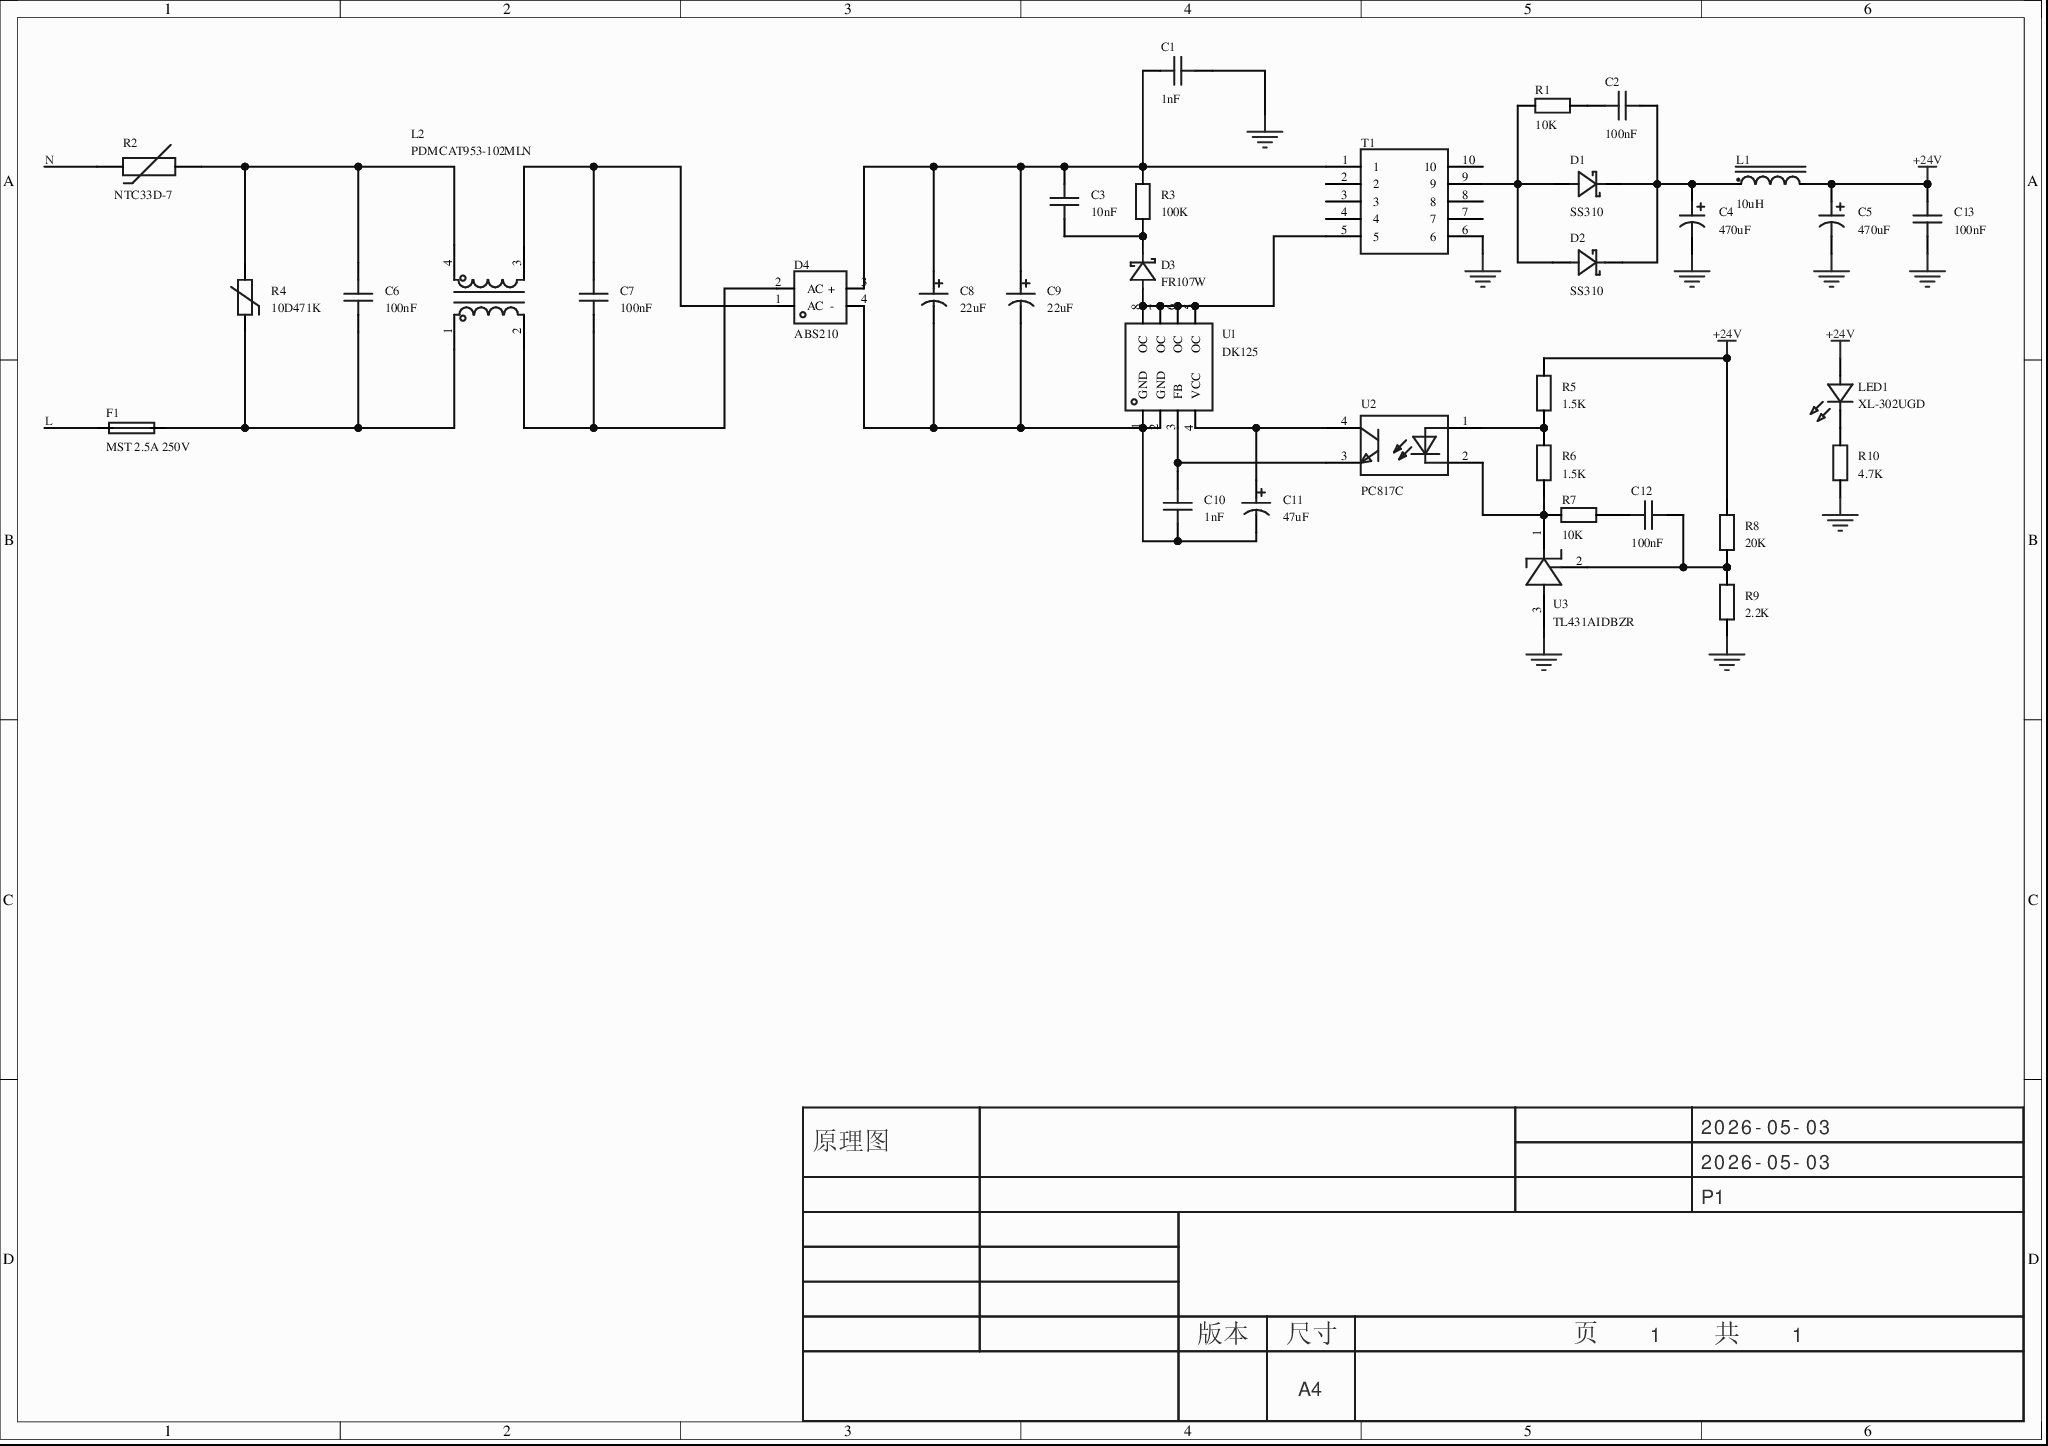
[diagram p0: MISC51479-3.schdoc]
# Altium project MISC51479-2.PrjPcb
1 sheet, 35 parts. Net scope: global (net labels, ports and power ports of the same name join across sheets).
Board file: MISC51479.pcbdoc

## Sheet MISC51479-3.schdoc
size 297 x 209 mm; Version: V1.0; @Project Name: MISC51479; @Page Count: 1; @Update Date: 2026-05-03; @Create Date: 2026-05-03; @Schematic Name: MISC51479; @Page No: 1; @Create Time: 01:06:52; @Update Time: 01:06:58; @Board Name: MISC51479

### Parts
C1  1nF  [CAP-TH_L7.5-W4.5-P10.00-D0.6]
C2  100nF  [C0603]
C3  10nF  [C1206]
C4  470uF  [CAP-TH_BD8.0-P3.50-D0.6-FD]
C5  470uF  [CAP-TH_BD8.0-P3.50-D0.6-FD]
C6  100nF  [CAP-TH_L13.0-W6.0-P10.00-D0.6]
C7  100nF  [CAP-TH_L13.0-W6.0-P10.00-D0.6]
C8  22uF  [CAP-TH_BD10.0-P5.00-D1.0-FD]
C9  22uF  [CAP-TH_BD10.0-P5.00-D1.0-FD]
C10  1nF  [C0603]
C11  47uF  [CAP-TH_BD5.0-P2.00-D0.8-FD]
C12  100nF  [C0603]
C13  100nF  [C0603]
D1  SS310  [SMA_L4.3-W2.6-LS5.0-FD]
D2  SS310  [SMA_L4.3-W2.6-LS5.0-FD]
D3  FR107W  [SOD-123FL_L2.7-W1.8-LS3.8-RD]
D4  ABS210  [ABF_L5.1-W4.4-P4.00-LS6.2-BL]
F1  MST 2.5A 250V  [FUSE-TH_L8.4-W4.3-P5.08-D1.0]
L1  10uH  [IND-TH_BD8.0-P5.00-D0.7]
L2  PDMCAT953-102MLN  [IND-TH_4P-L12.0-W6.0_PDMCAT953-501MLN]
LED1  XL-302UGD  [LED-TH_BD3.8-P2.54-FD_GREEN]
R1  10K  [R0603]
R2  NTC33D-7  [RES-TH_L6.5-W5.0-P5.00-D0.6-S4.40]
R3  100K  [R1206]
R4  10D471K  [RES-TH_L11.0-W6.0-P7.50-D0.8-S3.00]
R5  1.5K  [R0603]
R6  1.5K  [R0603]
R7  10K  [R0603]
R8  20K  [R0603]
R9  2.2K  [R0603]
R10  4.7K  [R0603]
T1  (no value)  [EE25 5+5]
U1  DK125  [DIP-8_L9.2-W6.4-P2.54-LS7.6-BL]
U2  PC817C  [DIP-4_L4.6-W6.5-P2.54-LS7.6-BL]
U3  TL431AIDBZR  [SOT-23-3_L2.9-W1.6-P1.90-LS2.8-BR]

### Nets
+24V: C5.1 C13.2 L1.2 LED1.1(A) R5.2 R8.2
GND: C1.2 C4.2 C5.2 C13.1 R9.1 R10.1 T1.6 U3.3(ANODE)
L: F1.1
N: R2.1
NetC1_1: C1.1 C3.2 C8.1 C9.1 D4.3(+) R3.2 T1.1
NetC2_1: C2.1 R1.2
NetC2_2: C2.2 C4.1 D1.2(K) D2.2(K) L1.1
NetC3_1: C3.1 D3.1(K) R3.1
NetC6_1: C6.1 L2.4 R2.2 R4.2
NetC6_2: C6.2 F1.2 L2.1 R4.1
NetC7_1: C7.1 D4.1(AC) L2.3
NetC7_2: C7.2 D4.2(AC) L2.2
NetC8_2: C8.2 C9.2 C10.1 C11.2 D4.4(-) U1.1(GND) U1.2(GND)
NetC10_2: C10.2 U1.3(FB) U2.3(EM)
NetC11_1: C11.1 U1.4(VCC) U2.4(COL)
NetC12_1: C12.1 R8.1 R9.2 U3.2(REF)
NetC12_2: C12.2 R7.2
NetD1_1: D1.1(A) D2.1(A) R1.1 T1.9
NetD3_2: D3.2(A) T1.5 U1.5(OC) U1.6(OC) U1.7(OC) U1.8(OC)
NetLED1_2: LED1.2(K) R10.2
NetR5_1: R5.1 R6.2 U2.1(AN)
NetR6_1: R6.1 R7.1 U2.2(CAT) U3.1(CATHODE)

Not connected (* = marked no-connect by the designer): T1 2* 3* 4* 7* 8* 10

### Notes on the sheet
- 2026-05-03
- 原理图
- P1
- 版本
- 尺寸
- A4
- 页    1    共    1

### Library data of the parts
C1 = KY1102M400VAC70Y10093: 容值:1nF;精度:±20%;工作电压(AC):400V;防护等级:Y1;; Manufacturer: KNSCHA(科尼盛); AddInBom: yes; ModelId: 9383b9b23f884ae7b98244ec8344dac5; ModelTransform: 431.76158,177.165,0,0,0,0,0,0,-137.795; Tolerance: ±20%; Voltage(AC): 400V; Ratings: Y1; safety certification: UL；ENEC；VDE；CQC; Symbol: KY1102M400VAC70Y10093; Device: KY1102M400VAC70Y10093; LCSC Part Name: 1nF ±20% 400V 等级:Y1; SupplierPart: C2943996; ManufacturerPart: KY1102M400VAC70Y10093; Supplier Footprint: 插件,P=10mm; JLCPCB Part Class: 扩展库; Datasheet: https://atta.szlcsc.com/upload/public/pdf/source/20240902/B2C4860AD6BBA55A7E27F7C368C73C02.pdf; Supplier: LCSC; ConvertToPcb: yes; FootprintName: CAP-TH_L7.5-W4.5-P10.00-D0.6; ModelName: CAP-TH_L7.5-W4.5-P10.00-D0.6; Value: 1nF
C2 C3 C10 C12 C13 = CAP_0603: ConvertToPcb: yes; SymbolName: Capacitance; ModelId: ac125912035d415993ca9572d50418b1; ModelName: C0603_L1.6-W0.8-H0.8; ModelTransform: 62.992,31.496,0,0,0,0,0,0,0; Device: CAP_0603; AddInBom: yes; Supplier Footprint: 0603
  C2 C12 C13: FootprintName: C0603; Value: 100nF
  C3: Value: 10nF; FootprintName: C1206
  C10: Value: 1nF; FootprintName: C0603
C4 C5 = JBLH2471M035D140RLM 470UF 35V: 容值:470uF;精度:±20%;额定电压:35V;纹波电流:2.9A@100kHz;等效串联电阻(ESR):35mΩ@100kHz;; Manufacturer: DMBJ(振宝佳); AddInBom: yes; ModelId: a2c936ec27754f809f3966430e36f767; ModelName: CAP-TH_D8.0-H8.0-P3.50; ModelTransform: 314.96,314.862,0,180,0,0,0,0,-137.795; Tolerance: ±20%; Voltage Rating: 35V; Lifetime: 2000hrs@105℃; Symbol: JBLH2471M035D140RLM 470UF 35V; Device: JBLH2471M035D140RLM 470UF 35V; LCSC Part Name: 470uF ±20% 35V; SupplierPart: C19270680; ManufacturerPart: JBLH2471M035D140RLM 470UF 35V; Supplier Footprint: 插件,D8xL14mm; JLCPCB Part Class: 扩展库; Datasheet: https://item.szlcsc.com/datasheet/JBLH2471M035D140RLM%2520470UF%252035V/20537870.html; Supplier: LCSC; ConvertToPcb: yes; FootprintName: CAP-TH_BD8.0-P3.50-D0.6-FD; Value: 470uF; Ripple Current: 2.9A@100kHz; Equivalent Series Resistance(ESR): 35mΩ@100kHz; Diameter: 8mm; Height - Seated (Max): 14mm
C6 C7 = MPX104K31C3KN15600: 容值:100nF;精度:±10%;工作电压(AC):275V；310V；305V;防护等级:X2;; Manufacturer: KNSCHA(科尼盛); AddInBom: yes; ModelId: ab2ba9e918834f5e935e28a3e5a6a2b8; ModelName: CAP-TH_L13.0-W6.0-H12.0-P10.0; ModelTransform: 511.81,236.22,0,0,0,0,0,0,-137.795; Tolerance: ±10%; Ratings: X2; safety certification: UL；CUL；KC；ENEC；VDE；CQC; Symbol: MPX104K31C3KN15600; Device: MPX104K31C3KN15600; LCSC Part Name: 100nF ±10% 275V 305V 310V 等级:X2; SupplierPart: C489079; ManufacturerPart: MPX104K31C3KN15600; Supplier Footprint: 插件,P=10mm; JLCPCB Part Class: 扩展库; Datasheet: https://atta.szlcsc.com/upload/public/pdf/source/20200225/C489079_75CB6A5338414DC85C4C6073302579B5.pdf; Supplier: LCSC; ConvertToPcb: yes; FootprintName: CAP-TH_L13.0-W6.0-P10.00-D0.6; Value: 100nF; Voltage(AC): 275V；310V；305V; Operating Temperature: -40℃~+110℃
C8 C9 = ERK2GM220G16OT: 容值:22uF;精度:±20%;额定电压:400V;纹波电流:-;等效串联电阻(ESR):-;; Manufacturer: AISHI(艾华集团); AddInBom: yes; ModelId: 6ce78ce5315348e095d700085da75e48; ModelName: CAP-TH_D10.0-H16.0-P5.00; ModelTransform: 394.094,393.72252,0,0,0,0,0,0,-137.795; Tolerance: ±20%; Voltage Rating: 400V; Pin Spacing: 5mm; Lifetime: 2000hrs@105℃; Symbol: ERK2GM220G16OT; Device: ERK2GM220G16OT; LCSC Part Name: 22uF ±20% 400V CLEAR 专门用于充电器; SupplierPart: C106587; ManufacturerPart: ERK2GM220G16OT; Supplier Footprint: 插件,D10xL16mm; JLCPCB Part Class: 扩展库; Datasheet: https://item.szlcsc.com/datasheet/ERK2GM220G16OT/107803.html; Supplier: LCSC; ConvertToPcb: yes; FootprintName: CAP-TH_BD10.0-P5.00-D1.0-FD; Value: 22uF; Ripple Current: -; Equivalent Series Resistance(ESR): -; Diameter: 10mm; Height - Seated (Max): 16mm
C11 = KS476M025D07RR0VH2FP0: 容值:47uF;精度:±20%;额定电压:25V;; Manufacturer: Chengx(承兴); Symbol: 47uF 25V 5*7; AddInBom: yes; ModelId: edeeed87cbc746108d01291548c38636; ModelName: CAP-TH_D5.0×H7.0×P2.0; ModelTransform: 197.091,196.7911,0,0,0,0,0,0,-137.795; Tolerance: ±20%; Voltage Rating: 25V; Pin Spacing: 2mm; Lifetime: 1000hrs@105℃; Device: KS476M025D07RR0VH2FP0; LCSC Part Name: 47uF ±20% 25V; SupplierPart: C44586; ManufacturerPart: KS476M025D07RR0VH2FP0; Supplier Footprint: 插件,D5xL7mm; JLCPCB Part Class: 扩展库; Datasheet: https://item.szlcsc.com/datasheet/KS476M025D07RR0VH2FP0/45588.html; Supplier: LCSC; ConvertToPcb: yes; FootprintName: CAP-TH_BD5.0-P2.00-D0.8-FD; Value: 47uF; Diameter: 5mm; Height - Seated (Max): 7mm; Operating Temperature: -40℃~+105℃
D1 D2 = SS310_C7420364: 二极管配置:独立式;正向压降(Vf):850mV@3A;直流反向耐压(Vr):100V;整流电流:3A;; Manufacturer: R+O(宏嘉诚); AddInBom: yes; ModelId: 7e24bebe6cd74171ae8c9de6fc5b78aa; ModelTransform: 198.4248,103.5431,0,180,0,0,0,0,0; Diode Configuration: 独立式; Voltage - DC Reverse(Vr): 100V; Current - Rectified: 3A; Reverse Leakage Current (Ir): 50uA@100V; Operating Junction Temperature Range: -55℃~+150℃; Non-Repetitive Peak Forward Surge Current: 80A; Symbol: SS310_C7420364; Device: SS310_C7420364; LCSC Part Name: 电压:100V 电流:3A; SupplierPart: C7420364; ManufacturerPart: SS310; Supplier Footprint: SMA(DO-214AC); JLCPCB Part Class: 扩展库; Datasheet: https://item.szlcsc.com/datasheet/SS310/8397186.html; Supplier: LCSC; ConvertToPcb: yes; FootprintName: SMA_L4.3-W2.6-LS5.0-FD; ModelName: SMA_L4.3-W2.6-LS5.0-FD; Voltage - Forward(Vf@If): 850mV@3A
D3 = FR107W_C18199114: 二极管配置:独立式;正向压降(Vf):1.3V@1.0A;直流反向耐压(Vr):1kV;整流电流:1A;反向恢复时间(Trr):500ns;; Manufacturer: R+O(宏嘉诚); AddInBom: yes; ModelId: 86f9151e155e4fe2af0c4f2e0a80302e; ModelName: SOD-123FL_L2.8-W1.8-H1.1-LS3.6; ModelTransform: 141.732,70.866,0,180,0,0,0,0,0; Diode Configuration: 独立式; Voltage - DC Reverse(Vr): 1kV; Current - Rectified: 1A; Reverse Leakage Current (Ir): 2uA@1000V; Reverse Recovery Time (trr): 500ns; Operating Junction Temperature Range: -55℃~+150℃; Non-Repetitive Peak Forward Surge Current: 30A; Symbol: FR107W_C18199114; Device: FR107W_C18199114; LCSC Part Name: 耐压:1000V 电流:1A 反向恢复时间：500ns; SupplierPart: C18199114; ManufacturerPart: FR107W; Supplier Footprint: SOD-123FL; JLCPCB Part Class: 扩展库; Datasheet: https://item.szlcsc.com/datasheet/FR107W/19354346.html; Supplier: LCSC; ConvertToPcb: yes; FootprintName: SOD-123FL_L2.7-W1.8-LS3.8-RD; Voltage - Forward(Vf@If): 1.3V@1.0A
D4 = ABS210_C42406052: 正向压降(Vf):1V@1A;直流反向耐压(Vr):1kV;整流电流:2A;非重复峰值浪涌电流 (Ifsm):60A;; Manufacturer: R+O(宏嘉诚); AddInBom: yes; ModelId: d26de62a0ec4497f9836f9d57bcbc20d; ModelName: ABF_L5.1-W4.4-H1.1-LS6.2-P4.00; ModelTransform: 200.787,244.094,0,0,0,0,0,0,0; Voltage - Forward(Vf@If): 1V@1A; Voltage - DC Reverse(Vr): 1kV; Current - Rectified: 2A; Reverse Leakage Current (Ir): 5uA; Non-Repetitive Peak Forward Surge Current: 60A; Operating Junction Temperature Range: -55℃~+150℃; Symbol: ABS210_C42406052; Device: ABS210_C42406052; LCSC Part Name: 耐压:1000V 电流:2A; SupplierPart: C42406052; ManufacturerPart: ABS210; Supplier Footprint: ABS; JLCPCB Part Class: 扩展库; Datasheet: https://item.szlcsc.com/datasheet/ABS210/44376175.html; Supplier: LCSC; ConvertToPcb: yes; FootprintName: ABF_L5.1-W4.4-P4.00-LS6.2-BL
F1 = MST 2.5A 250V: 类型:-;额定电流:2.5A;; Manufacturer: CONQUER(功得); AddInBom: yes; ModelId: 19fde7e2e811427cb03b64563a39ce50; ModelName: FUSE-TH_L8.4-W4.3-H7.7-P5.08-D0.6; ModelTransform: 328.7395,169.291,0,0,0,0,0,0,-866.142; Symbol: MST 2.5A 250V; Device: MST 2.5A 250V; LCSC Part Name: 插件式保险丝; SupplierPart: C388803; ManufacturerPart: MST 2.5A 250V; Supplier Footprint: 插件; JLCPCB Part Class: 扩展库; Datasheet: https://item.szlcsc.com/datasheet/MST%25202.5A%2520250V/364131.html; Supplier: LCSC; ConvertToPcb: yes; FootprintName: FUSE-TH_L8.4-W4.3-P5.08-D1.0; Type: -; Current Rating: 2.5A
L1 = XR8*10-100K-L: 电感值:10uH;精度:±10%;类型:工字电感;; Manufacturer: XR(祥如); AddInBom: yes; ModelId: e2b574cc7e974f3699d90eb153ec8540; ModelTransform: 314.96,314.96,0,90,0,0,-0.005,0,-196.85; Tolerance: ±10%; Type: 工字电感; Symbol: XR8*10-100K-L; Device: XR8*10-100K-L; LCSC Part Name: XR8*10-100K-L; SupplierPart: C5380240; ManufacturerPart: XR8*10-100K-L; Supplier Footprint: 插件,D8xL10mm; JLCPCB Part Class: 扩展库; Datasheet: https://atta.szlcsc.com/upload/public/pdf/source/20230323/5B1EF07D34541228859A732D583EB55B.pdf; Supplier: LCSC; ConvertToPcb: yes; FootprintName: IND-TH_BD8.0-P5.00-D0.7; ModelName: IND-TH_BD8.0-P5.00-D0.7; Value: 10uH
L2 = PDMCAT953-102MLN: 通道数:2;电感@频率:1mH@1kHz;直流电阻(DCR):25mΩ;; Manufacturer: PROD(谱罗德); AddInBom: yes; ModelId: 5ce8953f27a24618895504837993674b; ModelTransform: 472.34091,239.99,0,0,0,0,0,0,-196.85; Number of Lines: 2; Current Rating: 1.5A; DC Resistance(DCR): 25mΩ; Symbol: PDMCAT953-102MLN; Device: PDMCAT953-102MLN; LCSC Part Name: 共模电感1mH 1.5A 25mΩMAX 953环 过EMC; SupplierPart: C5158067; ManufacturerPart: PDMCAT953-102MLN; Supplier Footprint: 插件; JLCPCB Part Class: 扩展库; Datasheet: https://atta.szlcsc.com/upload/public/pdf/source/20220920/90718629BFB021D2715AF2FDDA682A79.pdf; Supplier: LCSC; ConvertToPcb: yes; FootprintName: IND-TH_4P-L12.0-W6.0_PDMCAT953-501MLN; ModelName: IND-TH_4P-L12.0-W6.0_PDMCAT953-501MLN; Inductance @ Frequency: 1mH@1kHz
LED1 = XL-302UGD: 灯头类型:3mm圆形灯头;发光颜色:翠绿色;正向压降(Vf):3.6V;功率:70mW;正向电流:20mA;波长:520nm~530nm;透镜颜色:绿色透镜;色温:-;发光强度:3000mcd;发光角度:30°;载带方式:-;工作温度:-20℃~+85℃;; Manufacturer: XINGLIGHT(成兴光); AddInBom: yes; ModelId: c917953ee2724e1d8eea37a428b0e119; ModelTransform: 134.40603,149.41647,0,0,0,0,-7.874,0,-137.795; Illumination Color: 翠绿色; Voltage - Forward(Vf): 3.6V; Power(Watts): 70mW; Forward Current: 20mA; Peak Wavelength: 520nm; Lens Color: 绿色透镜; Viewing Angle: 30°; Symbol: XL-302UGD; Device: XL-302UGD; LCSC Part Name: 绿发翠绿短脚LED; SupplierPart: C2895476; ManufacturerPart: XL-302UGD; Supplier Footprint: 插件,D=3mm; JLCPCB Part Class: 扩展库; Datasheet: https://item.szlcsc.com/datasheet/XL-302UGD/3136191.html; Supplier: LCSC; ConvertToPcb: yes; FootprintName: LED-TH_BD3.8-P2.54-FD_GREEN; ModelName: LED-TH_BD3.8-P2.54-FD_GREEN; Lamp Holder Type: 3mm圆形灯头; Wavelength - Dominant: 520nm~530nm; Color Temperature: -; Luminous Intensity: 3000mcd; Mounting Style: -; Operating Temperature: -20℃~+85℃
R1 R5-R10 = Res_0603: ConvertToPcb: yes; SymbolName: 电阻; ModelId: fc143cca1e79419f9cd78b61e9279f08; ModelTransform: 31.8897,63.7794,0,90,0,0,0,0,0; Device: Res_0603; AddInBom: yes; Supplier Footprint: 0603; FootprintName: R0603; ModelName: R0603
  R1 R7: Value: 10K
  R5 R6: Value: 1.5K
  R8: Value: 20K
  R9: Value: 2.2K
  R10: Value: 4.7K
R2 = NTC33D-7: 阻值:33Ω;B值(25℃/50℃):2950K;功率:-;B值精度:-;最大稳态电流(25℃):500mA;; Manufacturer: RUILON(瑞隆源); Symbol: MF72-33D-7; AddInBom: yes; ModelId: f94128eeffba4550be0fa1fd5c516166; ModelName: RES-TH_L6.5-W5.0-H10.0-P5.00-D0.6-S5.00; ModelTransform: 255.881,220.472,0,0,0,0,0,0.005,-196.85; Resistance @ 25℃: 33Ω; B Constant (25℃/50℃): 2950K; Steady State Current (Max): 500mA; Dissipation Factor: 9mW/℃; Thermal Time Constant: 30s; Pitch: 5mm; Device: NTC33D-7; LCSC Part Name: 33Ω; SupplierPart: C9177; ManufacturerPart: NTC33D-7; Supplier Footprint: 插件,P=5mm; JLCPCB Part Class: 扩展库; Datasheet: https://item.szlcsc.com/datasheet/NTC33D-7/9701.html; Supplier: LCSC; ConvertToPcb: yes; FootprintName: RES-TH_L6.5-W5.0-P5.00-D0.6-S4.40; B Constant (25℃/75℃): -; B Constant (25℃/85℃): -; B Constant (25℃/100℃): -; Power(Watts): -; B Constant Tolerance: -; Operating Temperature: -40℃~+150℃
R3 = Res_0603: ConvertToPcb: yes; SymbolName: 电阻; ModelId: fc143cca1e79419f9cd78b61e9279f08; ModelName: R0603; ModelTransform: 31.8897,63.7794,0,90,0,0,0,0,0; Value: 100K; Device: Res_0603; AddInBom: yes; Supplier Footprint: 0603; FootprintName: R1206
R4 = 10D471K_C49072849: 压敏电压:470V;钳位电压:775V;工作电压(DC):385V;工作电压(AC):300V;; Manufacturer: R+O(宏嘉诚); AddInBom: yes; ModelId: 697754fab3614c3ebaac71c05a7e96f9; ModelTransform: 432.55299,236.66945,0,0,0,0,0,0.005,-196.85; Varistor Voltage: 470V; Clamping Voltage: 775V; Maximum DC Volts: 385V; Maximum AC Volts: 300V; Peak Current: 2.5kA; Energy: 74J; Rated Wattage: 400mW; Symbol: 10D471K_C49072849; Value: 10D471K; Device: 10D471K_C49072849; LCSC Part Name: 10D471K; ManufacturerPart: 10D471K; Supplier Footprint: 插件,P=7.5mm; JLCPCB Part Class: 扩展库; Datasheet: https://item.szlcsc.com/datasheet/10D471K/51445315.html; Supplier: LCSC; ConvertToPcb: yes; FootprintName: RES-TH_L11.0-W6.0-P7.50-D0.8-S3.00; ModelName: RES-TH_L11.0-W6.0-P7.50-D0.8-S3.00
T1 = EE25: AddInBom: yes; Device: EE25; ConvertToPcb: yes; SymbolName: EE25; FootprintName: EE25 5+5
U1 = DK125: 工作电压:4.5V~4.9V;开关频率:61kHz~69kHz;晶体管耐压:700V;; Manufacturer: DK(东科半导体); AddInBom: yes; ModelId: 0f67547f9f69422e93d8ef5b6ef310c7; ModelTransform: 358.267,309.999,0,0,0,0,-0.004,0.002,-125.984; Isolation: 隔离; Duty Cycle(Max): 70%; Voltage - Breakdown: 700V; Topology: 反激式; Feedback System: 副边反馈; Symbol: DK125; Device: DK125; LCSC Part Name: 24W交直流转换芯片; SupplierPart: C171868; ManufacturerPart: DK125; Supplier Footprint: DIP-8; JLCPCB Part Class: 扩展库; Datasheet: https://item.szlcsc.com/datasheet/DK125/183254.html; Supplier: LCSC; ConvertToPcb: yes; FootprintName: DIP-8_L9.2-W6.4-P2.54-LS7.6-BL; ModelName: DIP-8_L9.2-W6.4-P2.54-LS7.6-BL; Voltage - Supply: 4.5V~4.9V; Frequency - Switching: 61kHz~69kHz; Features: 欠压保护(UVP)；过热保护(OTP)；短路保护(SCP)；过压保护(OVP)；过流保护(OCP)；软启动; Operating Temperature: -25℃~+125℃
U2 = PC817C_C3025068: 输入类型:DC;正向压降(Vf):1.2V;输出电流:50mA;隔离电压(Vrms):5kV;直流反向耐压(Vr):6V;负载电压:35V;输出通道数:1;集射极饱和电压(VCE(sat)):100mV@1mA,20mA;; Manufacturer: GOODWORK(固得沃克); AddInBom: yes; ModelId: d5e3ed0c3a524ad38d6bff221ba6c376; ModelName: DIP-4_L4.6-W6.5-H3.5-LS7.62-P2.54; ModelTransform: 180.3146,311.8104,0,0,0,0,0,0,-118.11; Input type: DC; Output Type: 光电三极管; Voltage - Forward(Vf): 1.2V; Output Current: 50mA; Isolation Voltage(Vrms): 5kV; Reverse Voltage: 6V; Load Voltage: 35V; Number of Outputs: 1; Rise time: 6us@2mA,100Ω; Fall time: 5us; Current Transfer Ratio (CTR) Minimum: 200%; Current Transfer Ratio (CTR) Maximum/Saturation Value: 400%; Symbol: PC817C_C3025068; Device: PC817C_C3025068; LCSC Part Name: 光电晶体管光电耦合器; SupplierPart: C3025068; ManufacturerPart: PC817C; Supplier Footprint: DIP-4; JLCPCB Part Class: 扩展库; Datasheet: https://item.szlcsc.com/datasheet/PC817C/3554571.html; Supplier: LCSC; ConvertToPcb: yes; FootprintName: DIP-4_L4.6-W6.5-P2.54-LS7.6-BL; Vce Saturation(VCE(sat)): 100mV@1mA,20mA; Operating Temperature: -55℃~+110℃; Forward Current(If): 50mA
U3 = TL431AIDBZR: 输出类型:可调;输入电压:-;输出电压:2.495V~36V;输出电流:100mA;精度:±1%;; Manufacturer: TI(德州仪器); AddInBom: yes; ModelId: 89cb27a44ab2466697082bb9fd73a7d0; ModelName: SOT-23-3L_L2.9-W1.6-H1.1-LS2.8-P0.95; ModelTransform: 114.173,110.236,0,90,0,0,0,0,0; Output Type: 可调; Output Current: 100mA; Tolerance: ±1%; Reference Type: 并联; Minimum Cathode Current for Regulation: 700uA; Symbol: TL431AIDBZR; Device: TL431AIDBZR; LCSC Part Name: TL431AIDBZR; SupplierPart: C23892; ManufacturerPart: TL431AIDBZR; Supplier Footprint: SOT-23; JLCPCB Part Class: 扩展库; Datasheet: https://www.ti.com/cn/lit/gpn/tl431; Supplier: LCSC; ConvertToPcb: yes; FootprintName: SOT-23-3_L2.9-W1.6-P1.90-LS2.8-BR; Input Voltage: -; Output Voltage: 2.495V~36V; Temperature Coefficient: -; Supply Current: -; Noise - 1/10Hz to 10Hz: -; Noise - 10Hz to 10kHz: -; Operating Temperature: -40℃~+85℃@(Ta)